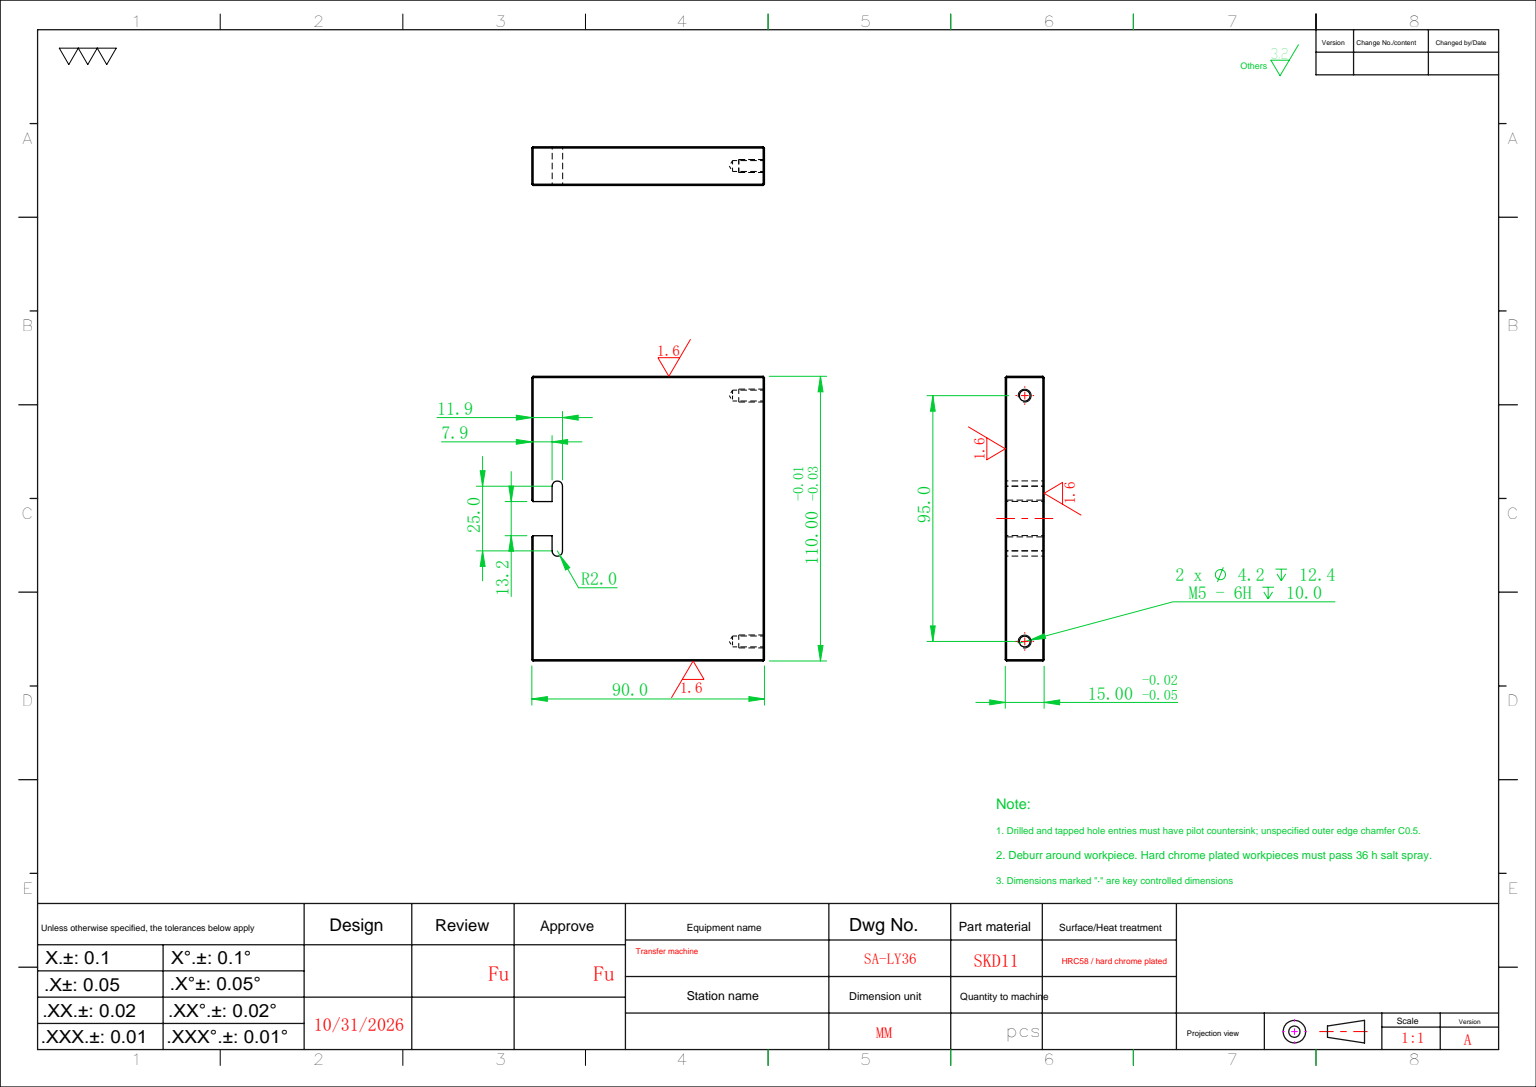
SolidWorks part; units mm, degrees
ref_plane "前视基准面" through (0, 0, 0) normal (0, 0, 1) x (1, 0, 0)
ref_plane "上视基准面" through (0, 0, 0) normal (0, 1, 0) x (1, 0, 0)
ref_plane "右视基准面" through (0, 0, 0) normal (1, 0, 0) x (0, 0, -1)
sketch "草图1" plane through (0, 0, 0) normal (0, 0, 1) x (1, 0, 0)
  line L1 (-55, -45) -> (55, -45)
  line L2 (-55, -45) -> (-55, 45)
  line L3 (-55, 45) -> (55, 45)
  line L4 (55, -45) -> (55, 45)
  line L5 (-55, -45) -> (55, 45) construction
  line L6 (-55, 45) -> (55, -45) construction
  point P0 (0, 0)
  dimension "D1" = 110
  dimension "D2" = 90
extrude "凸台-拉伸1" add sketch "草图1" along normal blind 15
sketch "草图2" plane through (0, 0, 15) normal (0, 0, 1) x (1, 0, 0)
  line L0 (55, 45) -> (-55, 45) construction
  line L1 (-6.6, 45) -> (6.6, 45)
  line L2 (-6.6, 45) -> (-6.6, 33.1)
  line L3 (-6.6, 33.1) -> (6.6, 33.1)
  line L4 (6.6, 45) -> (6.6, 33.1)
  line L5 (0, 0) -> (0, 67.7073) construction
  dimension "D1" = 13.2
  dimension "D2" = 11.9
extrude "切除-拉伸1" cut sketch "草图2" against normal through all and the other way through all
sketch "草图3" plane through (0, 0, 15) normal (0, 0, 1) x (1, 0, 0)
  line L0 (-12.5, 35.125) -> (12.5, 35.125) construction
  line L1 (-12.5, 37.15) -> (12.5, 37.15)
  line L2 (-12.5, 33.1) -> (12.5, 33.1)
  line L3 (6.6, 33.1) -> (-6.6, 33.1) construction
  line L4 (0, 33.1) -> (0, 39.2135) construction
  arc A0 (-12.5, 37.15) -> (-12.5, 33.1) centre (-12.5, 35.125) ccw
  arc A1 (12.5, 33.1) -> (12.5, 37.15) centre (12.5, 35.125) ccw
  point P2 (0, 35.125)
  dimension "D2" = 25
  dimension "D1" = 4.05
extrude "切除-拉伸2" cut sketch "草图3" against normal through all
hole_wizard "M5 螺纹孔1" positions "草图4" profile "草图5" tap size "M5" standard "ISO"
sketch "草图4" plane through (0, -45, 0) normal (0, -1, 0) x (-1, 0, 0)
  line L0 (0, 0) -> (0, -22.4051) construction
  line L2 (55, -7.5) -> (11.8515, -7.5) construction
  line L3 (55, -15) -> (55, 0) construction
  point P0 (-47.5, -7.5)
  point P2 (47.5, -7.5)
  dimension "D1" = 95
sketch "草图5" plane through (47.5, -45, 7.5) normal (1, 0, 0) x (0, 0, -1)
  line L0 (0, 0) -> (0, 13.6618)
  line L1 (0, 13.6618) -> (2.1, 12.4)
  line L2 (2.1, 12.4) -> (2.1, 0)
  line L5 (2.1, 0) -> (0, 0)
  line L10 (0, 13.6618) -> (-2.1, 12.4) construction
  line L11 (0, -6.35) -> (0, 107.95) construction
  dimension "螺纹孔钻头直径" = 4.2
  dimension "螺纹孔钻头深度" = 12.4
  dimension "导头角度" = 118
cosmetic thread "孔螺蚊线1"
cosmetic thread "孔螺蚊线2"
chamfer "倒角1" distance 0.5 angle 45 16 edges at (0, -45, 15) (30.8, 45, 15) (6.6, 45, 7.5) (30.8, 45, 0) (55, -45, 7.5) (55, 0, 15) (55, 45, 7.5) (55, 0, 0) (0, -45, 0) (-30.8, 45, 0) (-6.6, 45, 7.5) (-30.8, 45, 15) (-55, 45, 7.5) (-55, 0, 15) (-55, -45, 7.5) (-55, 0, 0)
